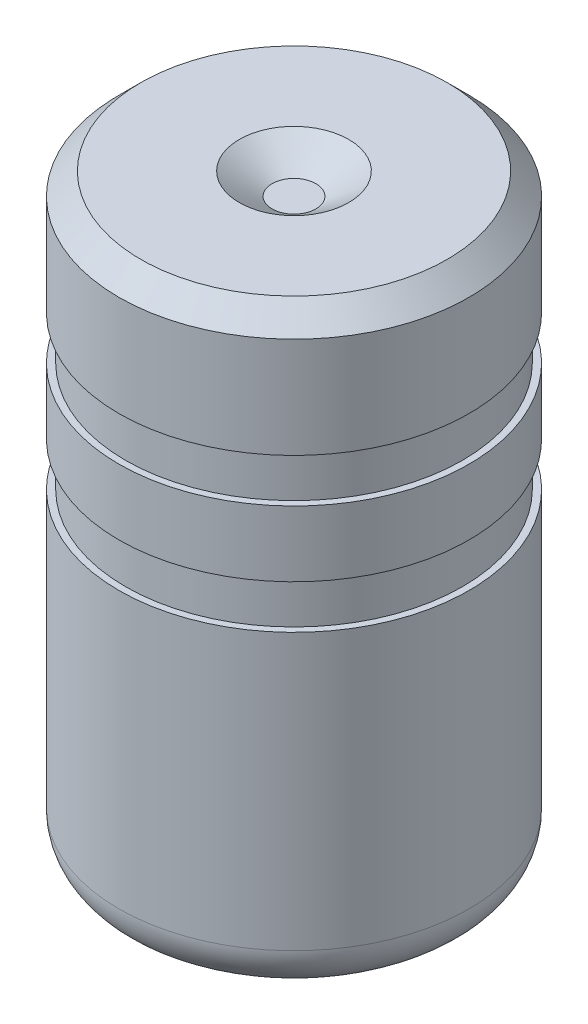
from build123d import *


with BuildPart() as part:
    # 草图1 → 旋转1 (revolve)
    with BuildSketch(Plane.XY, mode=Mode.PRIVATE) as revolve_1_sk:
        with BuildLine():
            Line((-3.25, 0), (-3.25, 12.5))
            Line((-3.25, 12.5), (0, 12.5))
            Line((0, 12.5), (0, 13.1))
            Line((0, 13.1), (-0.5, 13.1))
            Line((-0.5, 13.1), (-1.25, 13.6))
            Line((-1.25, 13.6), (-3.5, 13.6))
            Line((-3.5, 13.6), (-4, 13.1))
            Line((-4, 13.1), (-4, 10.8))
            Line((-4, 10.8), (-3.85, 10.8))
            Line((-3.85, 10.8), (-3.85, 9.8))
            Line((-3.85, 9.8), (-4, 9.8))
            Line((-4, 9.8), (-4, 8.3))
            Line((-4, 8.3), (-3.85, 8.3))
            Line((-3.85, 8.3), (-3.85, 7.3))
            Line((-3.85, 7.3), (-4, 7.3))
            Line((-4, 7.3), (-4, 1))
            ThreePointArc((-4, 1), (-3.791666667, 0.375), (-3.25, 0))
        make_face()
    revolve(revolve_1_sk.sketch.rotate(Axis((0, 0, 0), (0, 1, 0)), 270), axis=Axis((0, 0, 0), (0, 1, 0)))


solid = part.part
